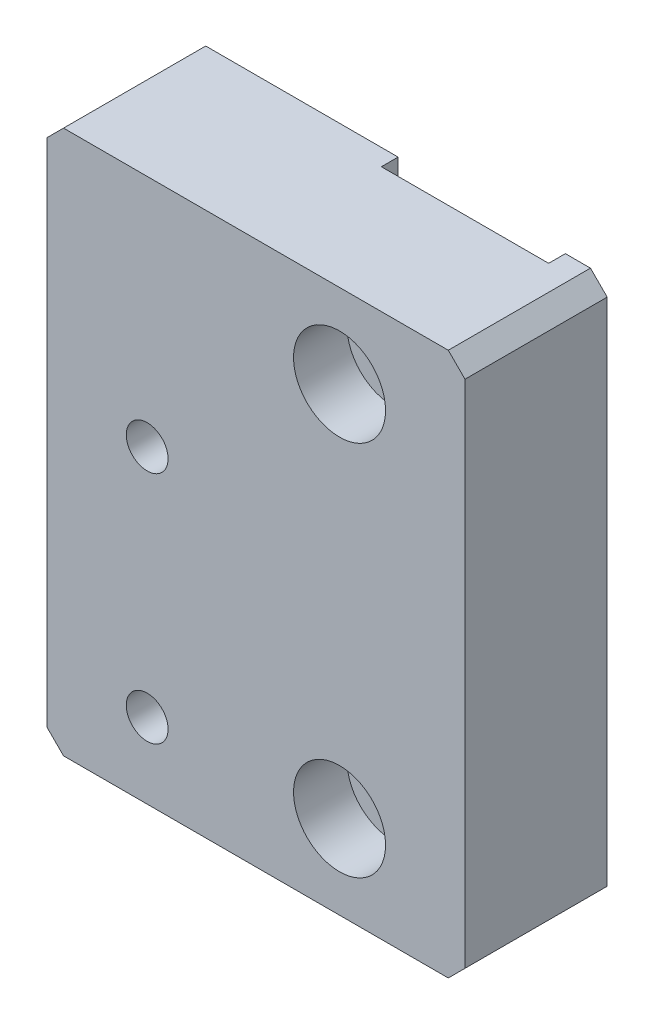
SolidWorks part; units mm, degrees
material "6061-T6"
ref_plane "前视基准面" through (0, 0, 0) normal (0, 0, 1) x (1, 0, 0)
ref_plane "上视基准面" through (0, 0, 0) normal (0, 1, 0) x (1, 0, 0)
ref_plane "右视基准面" through (0, 0, 0) normal (1, 0, 0) x (0, 0, -1)
sketch "草图2" plane through (0, 0, 0) normal (0, 0, 1) x (1, 0, 0)
  line L1 (0, 0) -> (50, 0)
  line L2 (0, 0) -> (0, -65)
  line L3 (0, -65) -> (50, -65)
  line L4 (50, 0) -> (50, -65)
  dimension "D1" = 65
  dimension "D2" = 50
extrude "凸台-拉伸1" add sketch "草图2" along normal blind 17
sketch "草图3" plane through (0, -65, 0) normal (0, -1, 0) x (1, 0, 0)
  line L0 (0, 0) -> (50, 0) construction
  line L1 (45, 0) -> (25, 0)
  line L2 (45, 0) -> (45, 2)
  line L3 (45, 2) -> (25, 2)
  line L4 (25, 0) -> (25, 2)
  line L5 (50, 17) -> (50, 0) construction
  dimension "D1" = 5
  dimension "D2" = 2
  dimension "D3" = 20
extrude "切除-拉伸1" cut sketch "草图3" against normal through all
chamfer "倒角1" distance 2 angle 45 4 edges at (50, -65, 8.5) (50, 0, 8.5) (0, 0, 8.5) (0, -65, 8.5)
hole_wizard "M6 螺纹孔1" positions "草图4" profile "草图5" tap size "M6" standard "ISO"
sketch "草图4" plane through (0, 0, 17) normal (0, 0, 1) x (1, 0, 0)
  line L0 (12, -56) -> (12, -28) construction
  line L2 (12, -42) -> (0, -42) construction
  line L7 (0, -2) -> (0, -63) construction
  line L8 (2, -65) -> (48, -65) construction
  point P0 (12, -28)
  point P2 (12, -56)
  dimension "D1" = 12
  dimension "D2" = 28
  dimension "D3" = 23
sketch "草图5" plane through (12, -28, 17) normal (1, 0, 0) x (0, -1, 0)
  line L0 (0, 0) -> (0, 18.5022)
  line L1 (0, 18.5022) -> (2.5, 17)
  line L2 (2.5, 17) -> (2.5, 0)
  line L5 (2.5, 0) -> (0, 0)
  line L10 (0, 18.5022) -> (-2.5, 17) construction
  line L11 (0, -6.35) -> (0, 107.95) construction
  dimension "螺纹孔钻头直径" = 5
  dimension "螺纹孔钻头深度" = 17
  dimension "导头角度" = 118
cosmetic thread "孔螺蚊线1" parameters "D1"=12, "D2"=6
cosmetic thread "孔螺蚊线2" parameters "D1"=12, "D2"=6
hole_wizard "M6 六角凹头螺钉的柱形沉头孔1" positions "草图6" profile "草图7" counterbore size "M6" standard "ISO"
sketch "草图6" plane through (0, 0, 17) normal (0, 0, 1) x (1, 0, 0)
  line L0 (35, -55) -> (35, -10) construction
  line L2 (25, -32.5) -> (45, -32.5) construction
  line L3 (25, 0) -> (25, -65) construction
  line L4 (45, 0) -> (45, -65) construction
  line L6 (35, -55) -> (35, -32.5) construction
  line L8 (35, -32.5) -> (50, -32.5) construction
  line L9 (50, -63) -> (50, -2) construction
  point P0 (35, -10)
  point P2 (35, -55)
  dimension "D1" = 45
sketch "草图7" plane through (35, -10, 17) normal (1, 0, 0) x (0, -1, 0)
  line L0 (0, 0) -> (0, 18.9828)
  line L1 (0, 18.9828) -> (3.3, 17)
  line L2 (3.3, 17) -> (3.3, 6.4)
  line L3 (3.3, 6.4) -> (5.5, 6.4)
  line L4 (5.5, 6.4) -> (5.5, 0)
  line L5 (5.5, 0) -> (0, 0)
  line L10 (0, 18.9828) -> (-3.3, 17) construction
  line L11 (0, -6.35) -> (0, 107.95) construction
  dimension "孔直径" = 6.6
  dimension "孔深度" = 17
  dimension "柱形沉头孔直径" = 11
  dimension "柱形沉头孔深度" = 6.4
  dimension "导头角度" = 118
